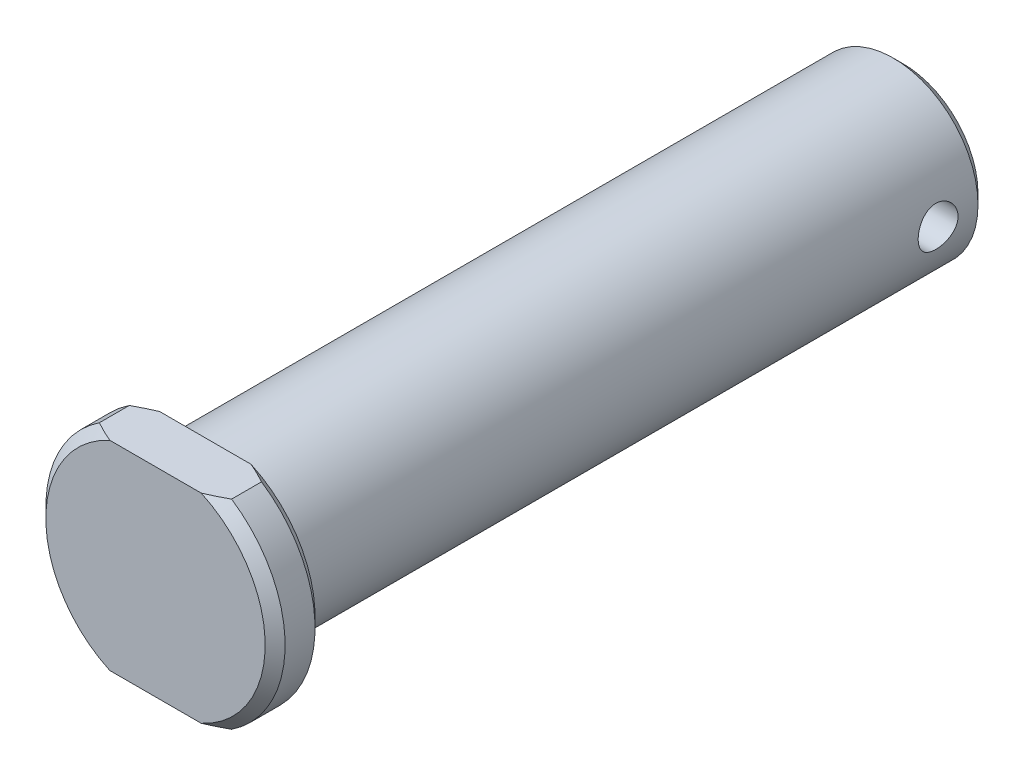
SolidWorks part; units mm, degrees
material "Q235B"
ref_plane "Front Plane" through (0, 0, 0) normal (0, 0, 1) x (1, 0, 0)
ref_plane "Top Plane" through (0, 0, 0) normal (0, 1, 0) x (1, 0, 0)
ref_plane "Right Plane" through (0, 0, 0) normal (1, 0, 0) x (0, 0, -1)
other "Configuration Table"
sketch "Sketch1" plane through (0, 0, 0) normal (1, 0, 0) x (0, 0, -1)
  line L0 (0, 11) -> (1, 12)
  line L1 (0, 0) -> (5, 0)
  line L2 (0, 0) -> (0, 11)
  line L3 (1, 12) -> (4, 12)
  line L4 (5, 0) -> (5, 11)
  line L5 (5, 0) -> (75, 0)
  line L6 (5, 0) -> (5, 8.5)
  line L7 (5, 8.5) -> (74, 8.5)
  line L8 (75, 0) -> (75, 7.5)
  line L9 (4, 12) -> (5, 11)
  line L10 (74, 8.5) -> (75, 7.5)
  point P1 (5, 12)
  point P2 (0, 12)
  point P5 (75, 8.5)
  dimension "D1" = 75
  dimension "D2" = 70
  dimension "D3" = 8.5
  dimension "D4" = 12
revolve "Revolve1" add sketch "Sketch1" angle 360 about L5
sketch "Sketch2" plane through (0, 0, 0) normal (1, 0, 0) x (0, 0, -1)
  line L0 (75, -7.5) -> (75, 7.5) construction
  circle A0 centre (70, 0) radius 2
  dimension "D1" = 5
  dimension "D2" = 4
extrude "Cut-Extrude1" cut sketch "Sketch2" against normal mid plane 20
sketch "Sketch3" plane through (0, 0, 0) normal (0, 0, 1) x (1, 0, 0)
  line L1 (-14.2806, 10) -> (13.0258, 10)
  line L2 (-14.2806, 10) -> (-14.2806, 18.0742)
  line L3 (-14.2806, 18.0742) -> (13.0258, 18.0742)
  line L4 (13.0258, 10) -> (13.0258, 18.0742)
  line L5 (-12.7667, -10) -> (14.0912, -10)
  line L6 (-12.7667, -10) -> (-12.7667, -18.1303)
  line L7 (-12.7667, -18.1303) -> (14.0912, -18.1303)
  line L8 (14.0912, -10) -> (14.0912, -18.1303)
  dimension "D1" = 20
  dimension "D2" = 10
extrude "Cut-Extrude2" cut sketch "Sketch3" against normal mid plane 10
fillet "Fillet1" radius 0.8 1 edges at (8.5, 0, -5)
